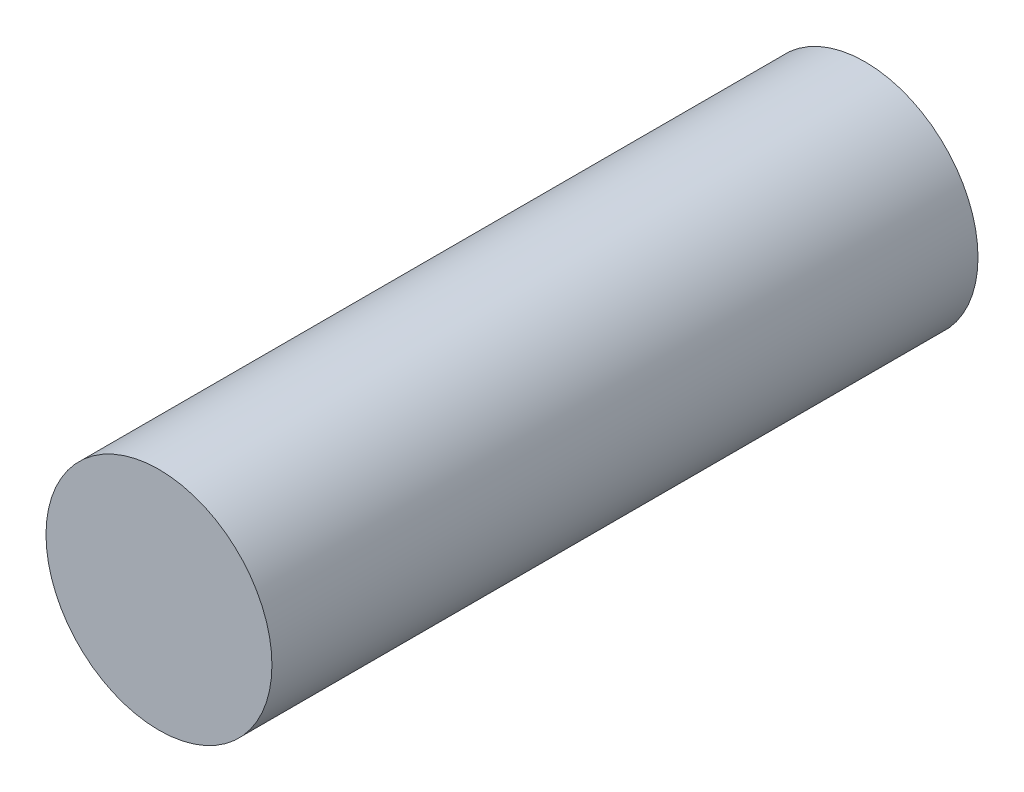
SolidWorks part; units mm, degrees
ref_plane "Front Plane" through (0, 0, 0) normal (0, 0, 1) x (1, 0, 0)
ref_plane "Top Plane" through (0, 0, 0) normal (0, 1, 0) x (1, 0, 0)
ref_plane "Right Plane" through (0, 0, 0) normal (1, 0, 0) x (0, 0, -1)
sketch "Sketch1" plane through (0, 0, 0) normal (0, 0, 1) x (1, 0, 0)
  circle A0 centre (0, 0) radius 4
extrude "Boss-Extrude1" add sketch "Sketch1" along normal blind 25
